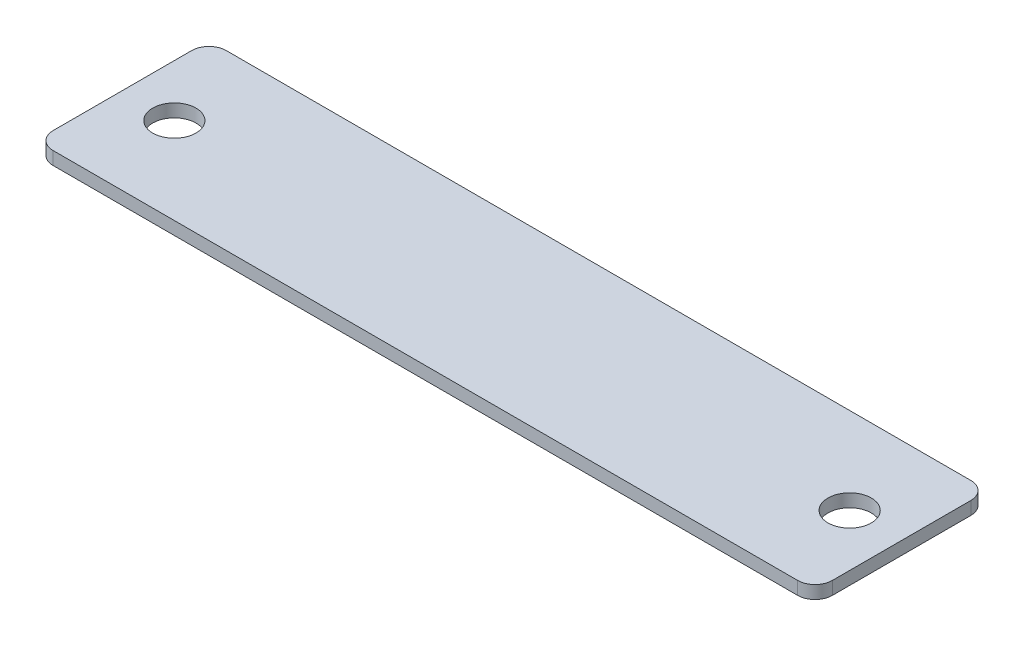
from build123d import *

# Parameters (mm, degrees)
SKETCH_1_W          = 90
SKETCH_1_H          = 20
EXTRUDE_1_DEPTH     = 1.5
SKETCH_2_R          = 2.5
CUT_EXTRUDE_1_DEPTH = 47.122120506
FILLET_1_R          = 2


with BuildPart() as part:
    # 草图1 → 凸台-拉伸1 (new body)
    with BuildSketch(Plane(origin=(0, 0, 0), x_dir=(1, 0, 0), z_dir=(0, 1, 0))):
        Rectangle(SKETCH_1_W, SKETCH_1_H)
    extrude(amount=EXTRUDE_1_DEPTH)

    # 草图2 → 切除-拉伸1 (cut, through all)
    with BuildSketch(Plane(origin=(0, 1.5, 0), x_dir=(1, 0, 0), z_dir=(0, 1, 0))):
        with Locations(Location((-39, 0, 0), (0, 0, 270))):
            Circle(SKETCH_2_R)
        with Locations(Location((39, 0, 0), (0, 0, 270))):
            Circle(SKETCH_2_R)
    extrude(amount=-CUT_EXTRUDE_1_DEPTH, mode=Mode.SUBTRACT)

    # 圆角1
    fillet_1_edges = [part.edges().sort_by_distance(p)[0] for p in [
        (45, 0.75, 10),
        (-45, 0.75, 10),
        (-45, 0.75, -10),
        (45, 0.75, -10),
    ]]
    fillet(fillet_1_edges, radius=FILLET_1_R)


solid = part.part
